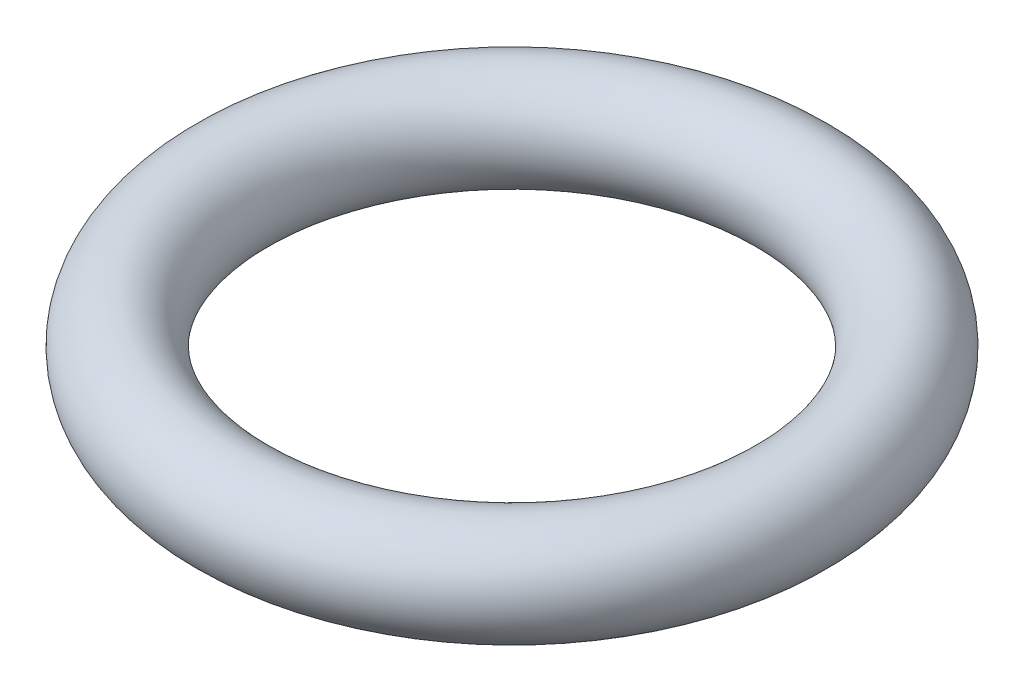
from build123d import *

# Parameters (mm, degrees)
SWEEP1_PROFILE_R = 0.92


with BuildPart() as part:
    # Sweep1: sweep along a path in Sketch1
    with BuildLine(Plane(origin=(0, 0, 0), x_dir=(1, 0, 0), z_dir=(0, 1, 0))) as sweep1_path:
        CenterArc((0, 0), 5.101647841, 0, 360)
    # Sweep1 profile (on start of the path) → Sweep1 (sweep)
    with BuildSketch(Plane(origin=(5.101647841, 0, 0), x_dir=(-1, 0, 0), z_dir=(0, 0, -1))):
        Circle(SWEEP1_PROFILE_R)
    sweep(path=sweep1_path.line)


solid = part.part
